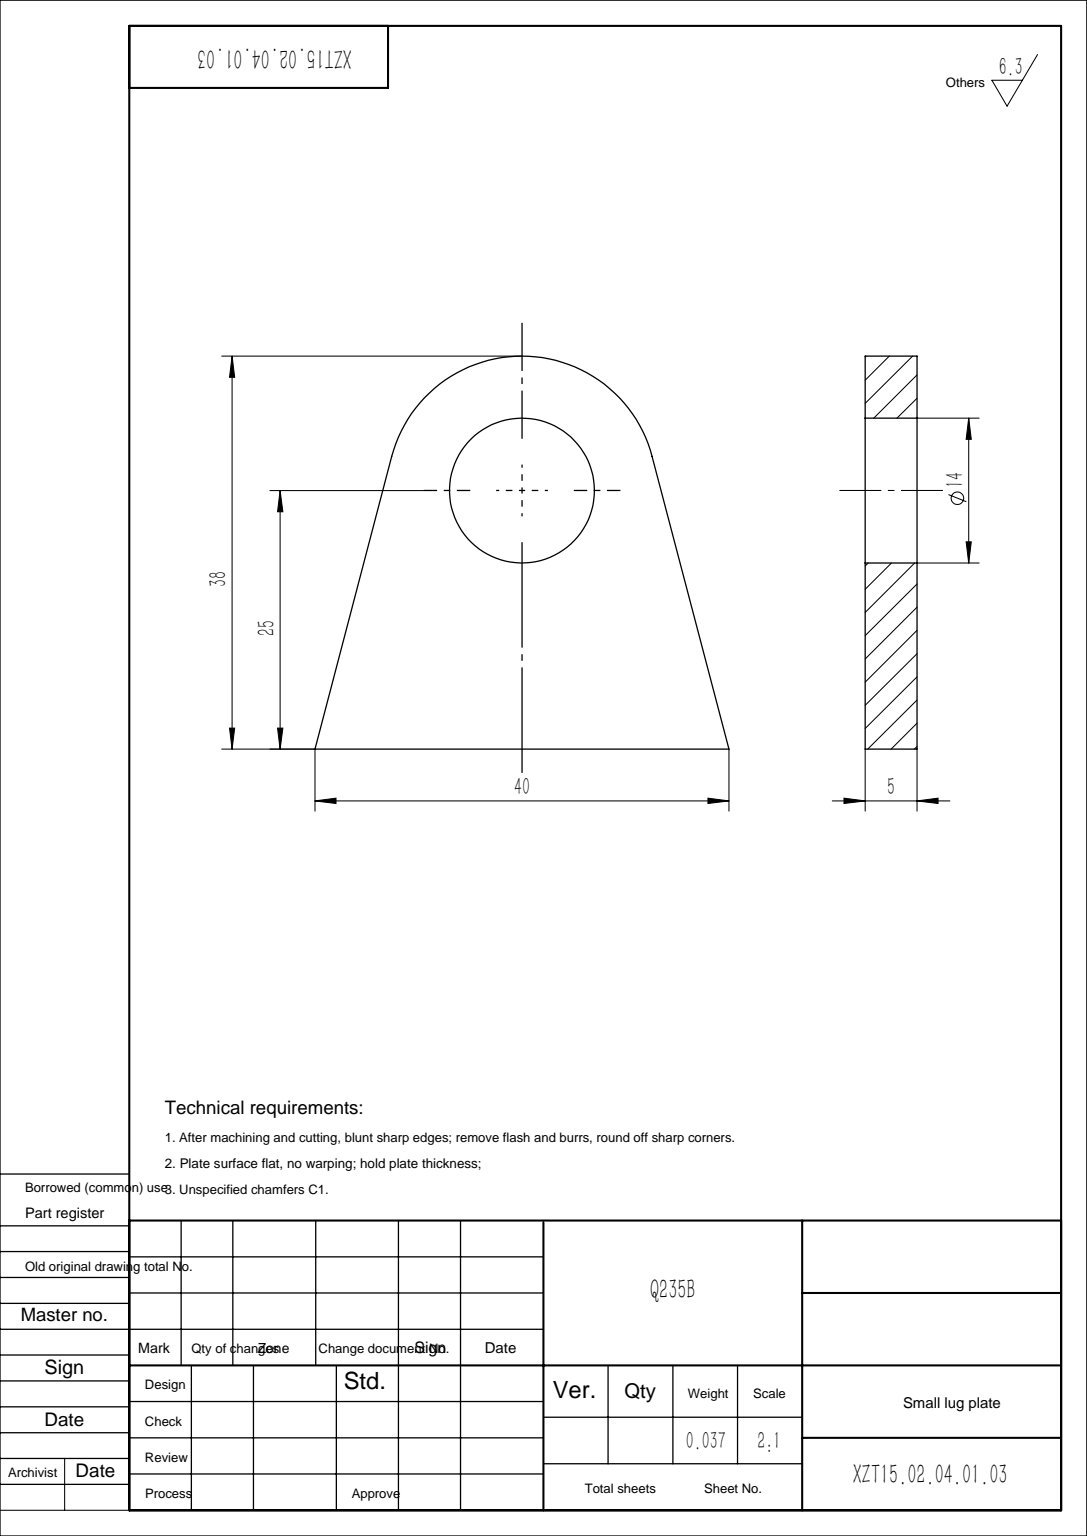
SolidWorks part; units mm, degrees
material "Q235B"
ref_plane "Front Plane" through (0, 0, 0) normal (0, 0, 1) x (1, 0, 0)
ref_plane "Top Plane" through (0, 0, 0) normal (0, 1, 0) x (1, 0, 0)
ref_plane "Right Plane" through (0, 0, 0) normal (1, 0, 0) x (0, 0, -1)
sketch "Sketch1" plane through (0, 0, 0) normal (0, 0, 1) x (1, 0, 0)
  line L0 (20, 0) -> (-20, 0)
  line L1 (-20, 0) -> (-12.5743, 28.2995)
  line L2 (0, 0) -> (0, 25) construction
  line L3 (20, 0) -> (12.5743, 28.2995)
  arc A0 (-12.5743, 28.2995) -> (12.5743, 28.2995) centre (0, 25) cw
  circle A1 centre (0, 25) radius 7
  dimension "D1" = 25
  dimension "D4" = 14
  dimension "D2" = 38
  dimension "D3" = 40
extrude "Boss-Extrude1" add sketch "Sketch1" along normal mid plane 5
